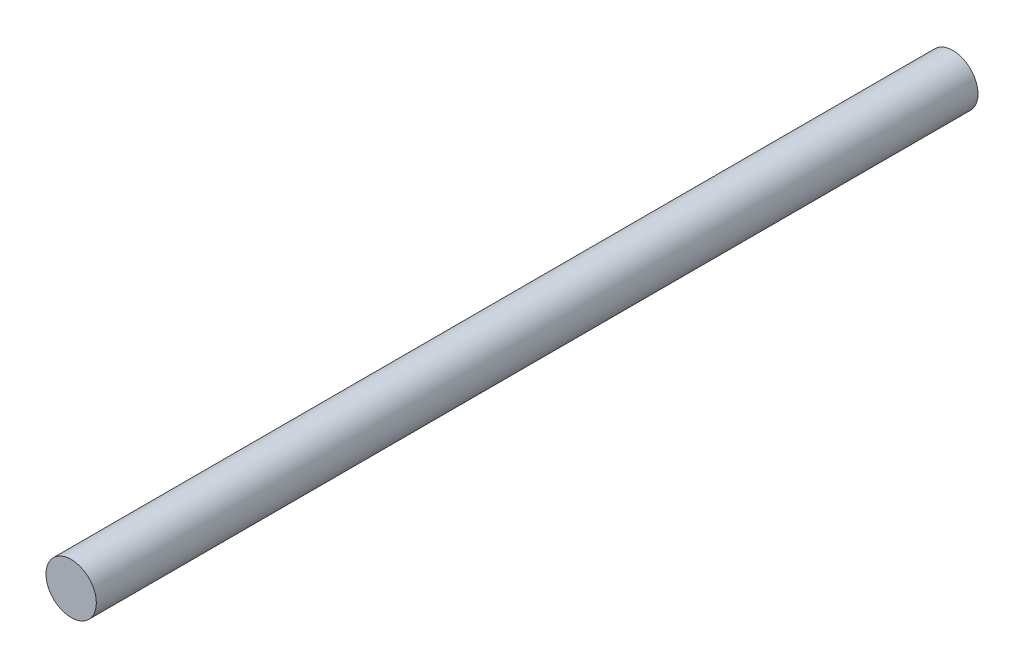
SolidWorks part; units mm, degrees
material "AISI 304"
ref_plane "前视基准面" through (0, 0, 0) normal (0, 0, 1) x (1, 0, 0)
ref_plane "上视基准面" through (0, 0, 0) normal (0, 1, 0) x (1, 0, 0)
ref_plane "右视基准面" through (0, 0, 0) normal (1, 0, 0) x (0, 0, -1)
sketch "草图1" plane through (0, 0, 0) normal (0, 0, 1) x (1, 0, 0)
  circle A0 centre (0, 0) radius 2
  dimension "D1" = 4
extrude "凸台-拉伸1" add sketch "草图1" along normal blind 70
